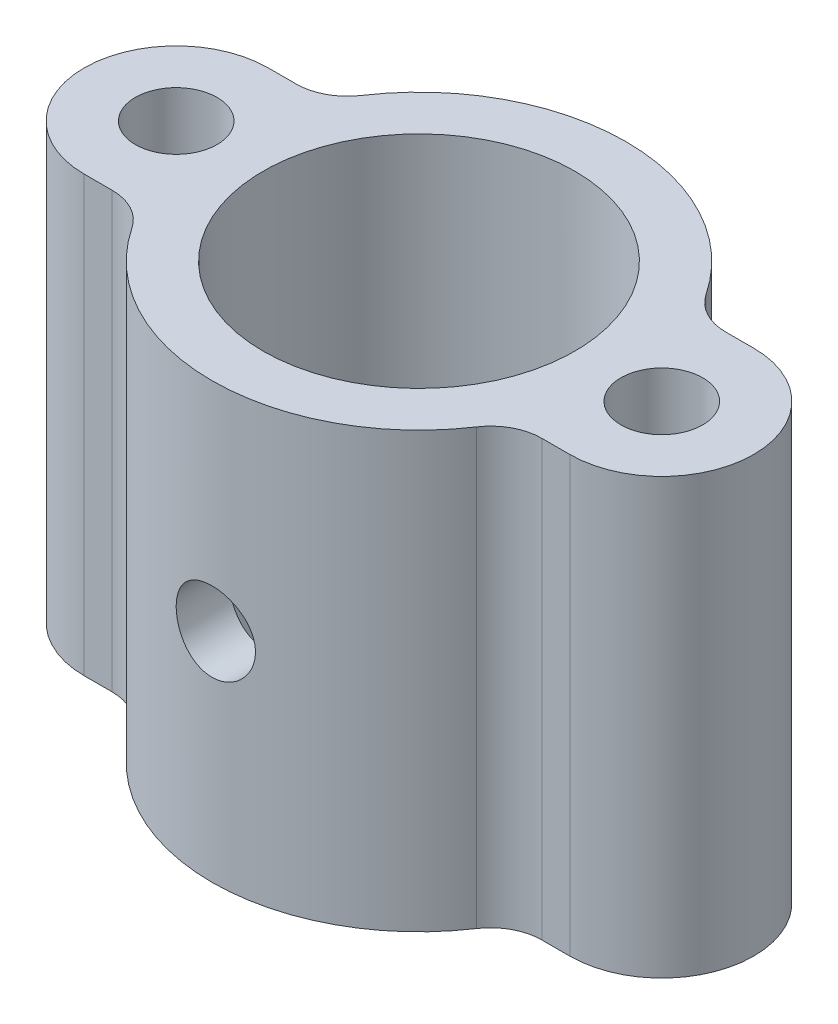
SolidWorks part; units mm, degrees
material "尼龙 101"
ref_plane "前视基准面" through (0, 0, 0) normal (0, 0, 1) x (1, 0, 0)
ref_plane "上视基准面" through (0, 0, 0) normal (0, 1, 0) x (1, 0, 0)
ref_plane "右视基准面" through (0, 0, 0) normal (1, 0, 0) x (0, 0, -1)
other "Configuration Table"
sketch "草图1" plane through (0, 0, 0) normal (0, 1, 0) x (1, 0, 0)
  line L0 (0, 0) -> (0, 15.2039) construction
  line L1 (0, 0) -> (14.2235, 0) construction
  line L2 (9.5, 3.6) -> (7.256, 3.6)
  line L3 (9.5, -3.6) -> (7.256, -3.6)
  line L4 (-9.5, -3.6) -> (-7.256, -3.6)
  line L5 (-9.5, 3.6) -> (-7.256, 3.6)
  circle A0 centre (0, 0) radius 6.1
  circle A2 centre (9.5, 0) radius 1.6
  arc A3 (9.5, -3.6) -> (9.5, 3.6) centre (9.5, 0) ccw
  arc A4 (-7.256, -3.6) -> (7.256, -3.6) centre (0, 0) ccw
  circle A5 centre (-9.5, 0) radius 1.6
  arc A6 (-9.5, -3.6) -> (-9.5, 3.6) centre (-9.5, 0) cw
  arc A7 (7.256, 3.6) -> (-7.256, 3.6) centre (0, 0) ccw
  circle A8 centre (9.5, 0) radius 2.75 construction
  dimension "D1" = 12.2
  dimension "D2" = 3.2
  dimension "D4" = 2
  dimension "D5" = 2
  dimension "D6" = 5.5
  dimension "D3" = 9.5
extrude "凸台-拉伸1" add sketch "草图1" along normal blind 17
fillet "圆角1" radius 2 4 edges at (-7.256, 8.5, -3.6) (7.256, 8.5, -3.6) (7.256, 8.5, 3.6) (-7.256, 8.5, 3.6)
sketch "草图2" plane through (0, 0, 0) normal (0, 0, 1) x (1, 0, 0)
  line L0 (0, 0) -> (0, 21.8602) construction
  line L1 (6.7409, 17) -> (-6.7409, 17) construction
  circle A0 centre (0, 8.5) radius 1.55
  dimension "D1" = 3.1
  dimension "D2" = 8.5
extrude "切除-拉伸1" cut sketch "草图2" against normal through all both and the other way through all
